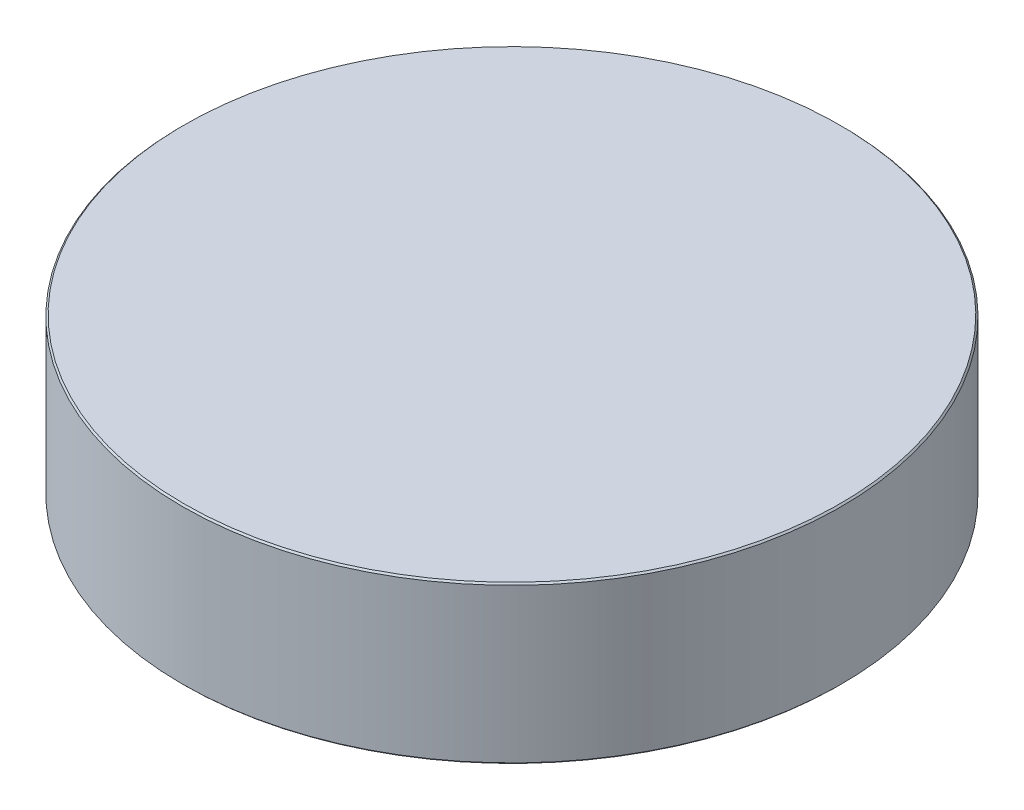
SolidWorks part; units mm, degrees
ref_plane "前视基准面" through (0, 0, 0) normal (0, 0, 1) x (1, 0, 0)
ref_plane "上视基准面" through (0, 0, 0) normal (0, 1, 0) x (1, 0, 0)
ref_plane "右视基准面" through (0, 0, 0) normal (1, 0, 0) x (0, 0, -1)
sketch "草图1" plane through (0, 0, 0) normal (0, 1, 0) x (1, 0, 0)
  circle A0 centre (0, 0) radius 210
  circle A1 centre (0, 0) radius 95.82
  dimension "D1" = 420
  dimension "D2" = 191.64
extrude "凸台-拉伸1" add sketch "草图1" along normal blind 100 contours A0 | A1
sketch "草图5" plane through (0, 100, 0) normal (0, 1, 0) x (1, 0, 0)
  circle A0 centre (0, 0) radius 150
extrude "凸台-拉伸4" add sketch "草图5" against normal blind 30
sketch "草图6" plane through (0, 0, 0) normal (0, -1, 0) x (1, 0, 0)
  circle A0 centre (0, 0) radius 185 construction
  point P2 (-185, 0)
  dimension "D1" = 370
hole_wizard "M10 螺纹孔1" positions "草图7" profile "草图8" tap size "M10" standard "GB"
sketch "草图7" plane through (0, 0, 0) normal (0, -1, 0) x (-1, 0, 0)
  circle A0 centre (0, 0) radius 185 construction
  point P0 (-185, 0)
sketch "草图8" plane through (185, 0, 0) normal (1, 0, 0) x (0, 0, -1)
  line L0 (0, 0) -> (0, 30.0537)
  line L1 (0, 30.0537) -> (4.25, 27.5)
  line L2 (4.25, 27.5) -> (4.25, 0.775)
  line L3 (4.25, 0.775) -> (5.025, 0)
  line L5 (5.025, 0) -> (0, 0)
  line L6 (-4.25, 0.775) -> (-5.025, 0) construction
  line L10 (0, 30.0537) -> (-4.25, 27.5) construction
  line L11 (0, -6.35) -> (0, 107.95) construction
  dimension "螺纹孔钻头直径" = 8.5
  dimension "螺纹孔钻头深度" = 27.5
  dimension "近端锥形沉头孔直径" = 10.05
  dimension "近端锥形沉头孔角度" = 90
  dimension "导头角度" = 118
pattern_circular "阵列(圆周)1" count 8 over 360 about axis through (0, 0, 0) along (0, 1, 0) of "M10 螺纹孔1"
chamfer "倒角1" distance 1 angle 45 3 edges at (0, 100, 210) (0, 0, 95.82) (0, 0, 210)
